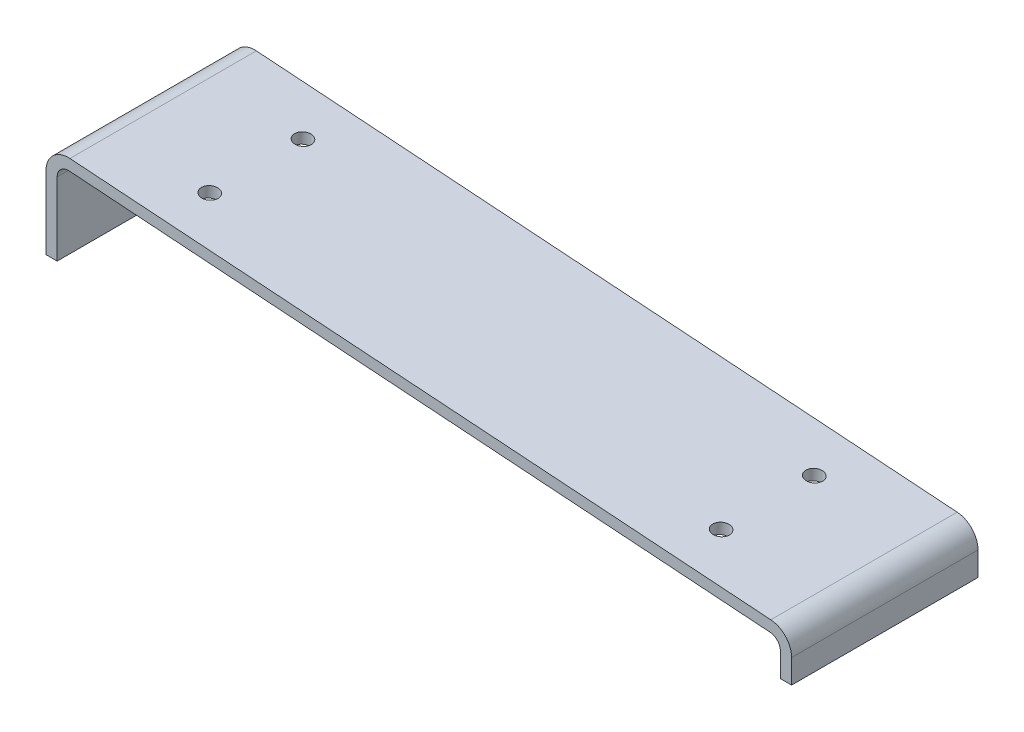
SolidWorks part; units mm, degrees
material "1023 carbon steel plate (SS)"
ref_plane "Front Plane" through (0, 0, 0) normal (0, 0, 1) x (1, 0, 0)
ref_plane "Top Plane" through (0, 0, 0) normal (0, 1, 0) x (1, 0, 0)
ref_plane "Right Plane" through (0, 0, 0) normal (1, 0, 0) x (0, 0, -1)
sketch "Sketch1" plane through (0, 0, 0) normal (0, 0, 1) x (1, 0, 0)
  line L0 (0, 0) -> (0, -52)
  line L2 (400, -52) -> (400, -28)
  line L3 (0, 0) -> (400, -28)
  line L4 (6, -6.4347) -> (6, -52)
  line L5 (6, -6.4347) -> (394, -33.5947)
  line L6 (394, -52) -> (394, -33.5947)
  line L7 (6, -52) -> (0, -52)
  line L8 (394, -52) -> (400, -52)
  dimension "D1" = 52
  dimension "D2" = 400
  dimension "D3" = 24
  dimension "D4" = 6
extrude "Boss-Extrude1" add sketch "Sketch1" along normal blind 100 contours L8 L2 L3 L0 L7 L4 L5 L6
sketch "Sketch4" plane through (0, 0, 0) normal (0.0698, 0.9976, 0) x (0.9976, -0.0698, 0)
  line L0 (0, 0) -> (400.9788, 0) construction
  line L1 (0, -100) -> (0, 0) construction
  circle A0 centre (63, -25) radius 4.5
  circle A1 centre (338, -25) radius 4.5
  circle A2 centre (63, -75) radius 4.5
  circle A3 centre (338, -75) radius 4.5
  dimension "D4" = 9
  dimension "D5" = 50
  dimension "D1" = 275
  dimension "D2" = 25
  dimension "D3" = 63
extrude "Cut-Extrude2" cut sketch "Sketch4" against normal blind 100
fillet "Fillet1" radius 12 2 edges at (400, -28, 50) (0, 0, 50)
fillet "Fillet2" radius 6 2 edges at (394, -33.5947, 50) (6, -6.4347, 50)
